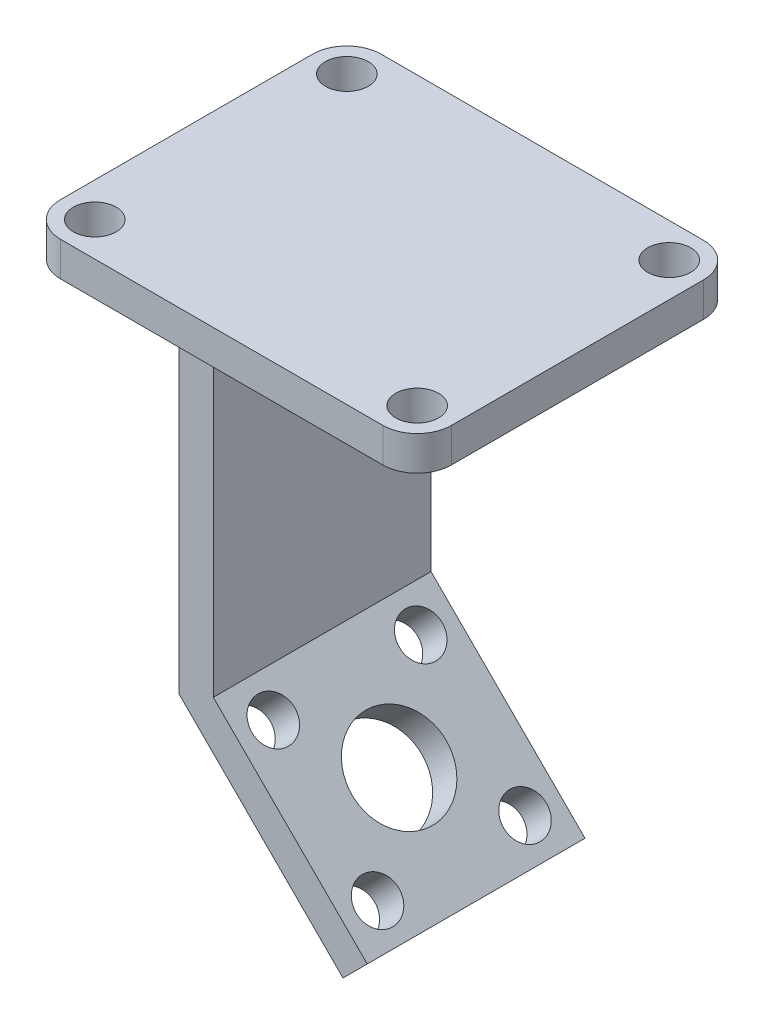
SolidWorks part; units mm, degrees
ref_plane "Front Plane" through (0, 0, 0) normal (0, 0, 1) x (1, 0, 0)
ref_plane "Top Plane" through (0, 0, 0) normal (0, 1, 0) x (1, 0, 0)
ref_plane "Right Plane" through (0, 0, 0) normal (1, 0, 0) x (0, 0, -1)
sketch "Sketch1" plane through (0, 0, 0) normal (0, 0, 1) x (1, 0, 0)
  line L0 (51.1656, 84.9757) -> (42.1853, 93.9559)
  line L1 (42.1853, 93.9559) -> (42.1853, 113.634)
extrude "Extrude-Thin1" add sketch "Sketch1" against normal blind 12.7 thin thin type one direction reverse wall 2
sketch "Sketch3" plane through (0, 113.634, 0) normal (0, 1, 0) x (1, 0, 0)
  line L0 (51.1656, 6.35) -> (40.1853, 6.35) construction
  line L5 (51.1656, 12.7) -> (51.1656, 0) construction
  line L7 (40.1853, 12.7) -> (40.1853, 0) construction
  line L8 (40.1853, 6.35) -> (45.6754, 6.35) construction
  line L9 (45.6754, 6.35) -> (45.6754, 13.9713) construction
  line L11 (57.0754, 15.7) -> (34.2754, 15.7)
  line L12 (57.0754, 15.7) -> (57.0754, -3)
  line L13 (57.0754, -3) -> (34.2754, -3)
  line L14 (34.2754, 15.7) -> (34.2754, -3)
  dimension "D1" = 5.9099
  dimension "D2" = 22.8
  dimension "D3" = 18.7
extrude "Boss-Extrude2" add sketch "Sketch3" along normal blind 2 separate body
fillet "Fillet1" radius 2 4 edges at (57.0754, 114.634, 3) (34.2754, 114.634, 3) (34.2754, 114.634, -15.7) (57.0754, 114.634, -15.7)
sketch "Sketch4" plane through (0, 115.634, 0) normal (0, 1, 0) x (1, 0, 0)
  circle A0 centre (55.0754, 13.7) radius 1.25
  circle A1 centre (55.0754, -1) radius 1.25
  circle A2 centre (36.2754, -1) radius 1.25
  circle A3 centre (36.2754, 13.7) radius 1.25
  dimension "D1" = 2.5
extrude "Cut-Extrude1" cut sketch "Sketch4" against normal blind 2
sketch "Sketch5" plane through (68.0706, 68.0706, 0) normal (0.7071, 0.7071, 0) x (0, 0, -1)
  circle A0 centre (6.35, 30.2574) radius 2.75
  dimension "D1" = 5.5
extrude "Cut-Extrude2" cut sketch "Sketch5" against normal through all both and the other way through all
sketch "Sketch6" plane through (66.6564, 66.6564, 0) normal (-0.7071, -0.7071, 0) x (0, 0, 1)
  circle A0 centre (-10.65, 34.5574) radius 1.25
  circle A1 centre (-2.05, 34.5574) radius 1.25
  circle A2 centre (-2.05, 25.9574) radius 1.25
  circle A3 centre (-10.65, 25.9574) radius 1.25
  dimension "D1" = 2.5
extrude "Cut-Extrude3" cut sketch "Sketch6" against normal blind 10
